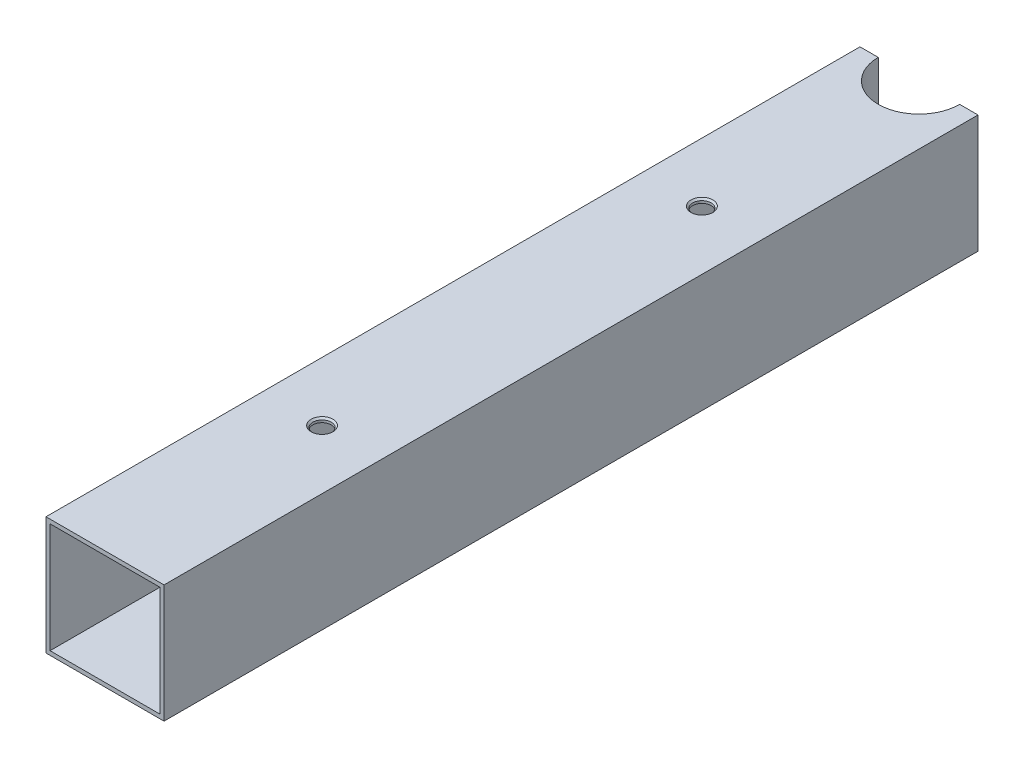
SolidWorks part; units mm, degrees
ref_plane "Front Plane" through (0, 0, 0) normal (0, 0, 1) x (1, 0, 0)
ref_plane "Top Plane" through (0, 0, 0) normal (0, 1, 0) x (1, 0, 0)
ref_plane "Right Plane" through (0, 0, 0) normal (1, 0, 0) x (0, 0, -1)
other "Configuration Table"
sketch "Sketch1" plane through (0, 0, 0) normal (0, 0, 1) x (1, 0, 0)
  line L0 (-42, 42) -> (1.5, 42)
  line L1 (-40.5, 40.5) -> (0, 40.5)
  line L2 (-40.5, 40.5) -> (-40.5, 0)
  line L3 (-40.5, 0) -> (0, 0)
  line L4 (0, 40.5) -> (0, 0)
  line L5 (1.5, 42) -> (1.5, -1.5)
  line L6 (-42, -1.5) -> (1.5, -1.5)
  line L7 (-42, 42) -> (-42, -1.5)
  dimension "D1" = 40.5
  dimension "D2" = 40.5
  dimension "D3" = 1.5
extrude "Boss-Extrude1" add sketch "Sketch1" along normal blind 300
sketch "Sketch2" plane through (0, 0, 0) normal (0, 0, -1) x (-1, 0, 0)
  line L1 (-1.5, 42) -> (42, 42)
  line L2 (-1.5, 42) -> (-1.5, -1.5)
  line L3 (-1.5, -1.5) -> (42, -1.5)
  line L4 (42, 42) -> (42, -1.5)
extrude "Boss-Extrude2" add sketch "Sketch2" against normal blind 30
sketch "Sketch3" plane through (0, 42, 0) normal (0, 1, 0) x (1, 0, 0)
  line L0 (-20.25, 0) -> (-20.25, -300) construction
  line L1 (1.5, 0) -> (-42, 0) construction
  line L2 (1.5, -300) -> (-42, -300) construction
  line L3 (-42, -150) -> (1.5, -150) construction
  line L4 (-42, -300) -> (-42, 0) construction
  line L5 (1.5, -300) -> (1.5, 0) construction
  circle A0 centre (-20.25, -80) radius 5
  circle A1 centre (-20.25, -220) radius 5
  point P12 (-20.25, -80)
  point P14 (-20.25, -220)
  dimension "D1" = 10
  dimension "D2" = 70
hole_wizard "M8 Tapped Hole1" positions "Sketch3" profile "Sketch4" tap size "M8" standard "GB" end condition through all
sketch "Sketch4" plane through (-20.25, 42, 220) normal (1, 0, 0) x (0, 0, 1)
  line L0 (0, 0) -> (0, 43.5)
  line L1 (0, 43.5) -> (3.4, 43.5)
  line L2 (3.4, 43.5) -> (3.4, 0.625)
  line L3 (3.4, 0.625) -> (4.025, 0)
  line L5 (4.025, 0) -> (0, 0)
  line L6 (-3.4, 0.625) -> (-4.025, 0) construction
  line L11 (0, -6.35) -> (0, 107.95) construction
  dimension "通孔螺纹孔钻头直径" = 6.8
  dimension "通孔螺纹孔钻头深度" = 43.5
  dimension "近端锥形沉头孔直径" = 8.05
  dimension "近端锥形沉头孔角度" = 90
cosmetic thread "Cosmetic thread 1" parameters "D2"=8
cosmetic thread "Cosmetic thread 2" parameters "D2"=8
sketch "Sketch5" plane through (0, 42, 0) normal (0, 1, 0) x (1, 0, 0)
  line L0 (-20.25, 0) -> (-20.25, -300) construction
  line L1 (1.5, 0) -> (-42, 0) construction
  line L2 (1.5, -300) -> (-42, -300) construction
  line L3 (1.5, -150) -> (-42, -150)
  line L4 (1.5, -300) -> (1.5, 0) construction
  line L5 (-42, -300) -> (-42, 0) construction
  line L6 (-35.25, 0) -> (-5.25, 0)
  arc A0 (-35.25, 0) -> (-5.25, 0) centre (-20.25, 0) ccw
  dimension "D1" = 15
extrude "Cut-Extrude1" cut sketch "Sketch5" against normal through all contours L6 A0
ref_plane "Plane2" through (0, 0, 0) normal (0, 0, -1) x (-1, 0, 0)
sketch "Sketch6" plane through (0, 0, 0) normal (0, 0, -1) x (-1, 0, 0)
  line L0 (5.25, 20.25) -> (35.25, 20.25) construction
  line L1 (5.25, -1.5) -> (5.25, 42) construction
  line L2 (35.25, -1.5) -> (35.25, 42) construction
  line L3 (20.25, 31.9498) -> (20.25, -1.5) construction
  line L4 (5.25, -1.5) -> (35.25, -1.5) construction
  circle A0 centre (20.25, 20.25) radius 5
extrude "Cut-Extrude2" cut sketch "Sketch6" against normal through all
